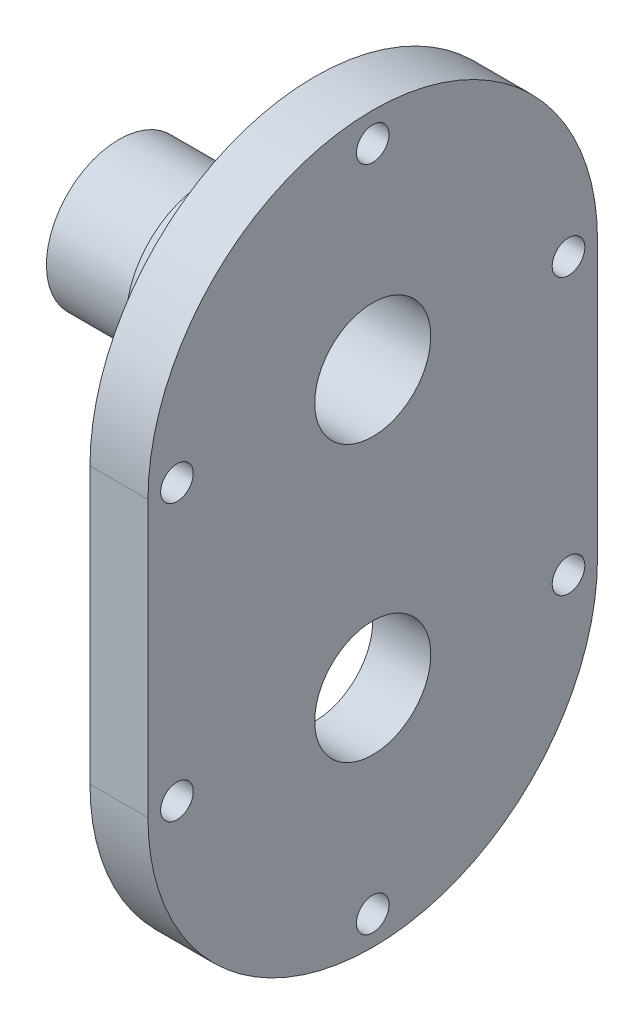
from build123d import *

# Parameters (mm, degrees)
BOSS_EXTRUDE1_DEPTH                  = 8
F_16_0_16_DIAMETER_HOLE1_D           = 16
F_16_0_16_DIAMETER_HOLE2_D           = 16
F_16_0_16_DIAMETER_HOLE2_CSINK_D     = 19.6
F_16_0_16_DIAMETER_HOLE2_CSINK_ANGLE = 90
F_4_5_4_5_DIAMETER_HOLE1_D           = 4.5
CHAMFER1_SIZE                        = 1.5


with BuildPart() as part:
    # Sketch1 → Boss-Extrude1 (new body)
    with BuildSketch(Plane(origin=(8, 0, 0), x_dir=(0, 0, -1), z_dir=(1, 0, 0))):
        with BuildLine():
            Line((31, -19), (31, 19))
            ThreePointArc((31, 19), (0, 50), (-31, 19))
            Line((-31, 19), (-31, -19))
            ThreePointArc((-31, -19), (0, -50), (31, -19))
        make_face()
    extrude(amount=-BOSS_EXTRUDE1_DEPTH)

    # Sketch2 → Revolve1 (revolve)
    with BuildSketch(Plane.XY):
        Polygon((-27, 29), (-27, 19), (0, 19), (0, 30.786116689), (-15, 30), (-15, 29), align=None)
    revolve(axis=Axis((-27, 19, 0), (1, 0, 0)))

    # Ø16.0 (16) Diameter Hole1 (through all)
    with Locations(Plane.ZY):
        with Locations((0, -19)):
            Hole(F_16_0_16_DIAMETER_HOLE1_D / 2)

    # Ø16.0 (16) Diameter Hole2 (through all)
    with Locations(Plane.ZY.offset(27)):
        with Locations((0, 19)):
            CounterSinkHole(F_16_0_16_DIAMETER_HOLE2_D / 2, F_16_0_16_DIAMETER_HOLE2_CSINK_D / 2, counter_sink_angle=F_16_0_16_DIAMETER_HOLE2_CSINK_ANGLE)

    # Ø4.5 (4.5) Diameter Hole1 (through all)
    with Locations(Plane.ZY):
        with Locations((0, 46), (27, 19), (-27, 19), (27, -19), (-27, -19), (0, -46)):
            Hole(F_4_5_4_5_DIAMETER_HOLE1_D / 2)

    # Chamfer1
    chamfer1_edges = [part.edges().sort_by_distance(p)[0] for p in [
        (0, -46, 2.25),
        (0, -19, -24.75),
        (0, -19, 29.25),
        (0, 19, -24.75),
        (0, 19, 29.25),
        (0, 46, 2.25),
    ]]
    chamfer(chamfer1_edges, length=CHAMFER1_SIZE)


solid = part.part
